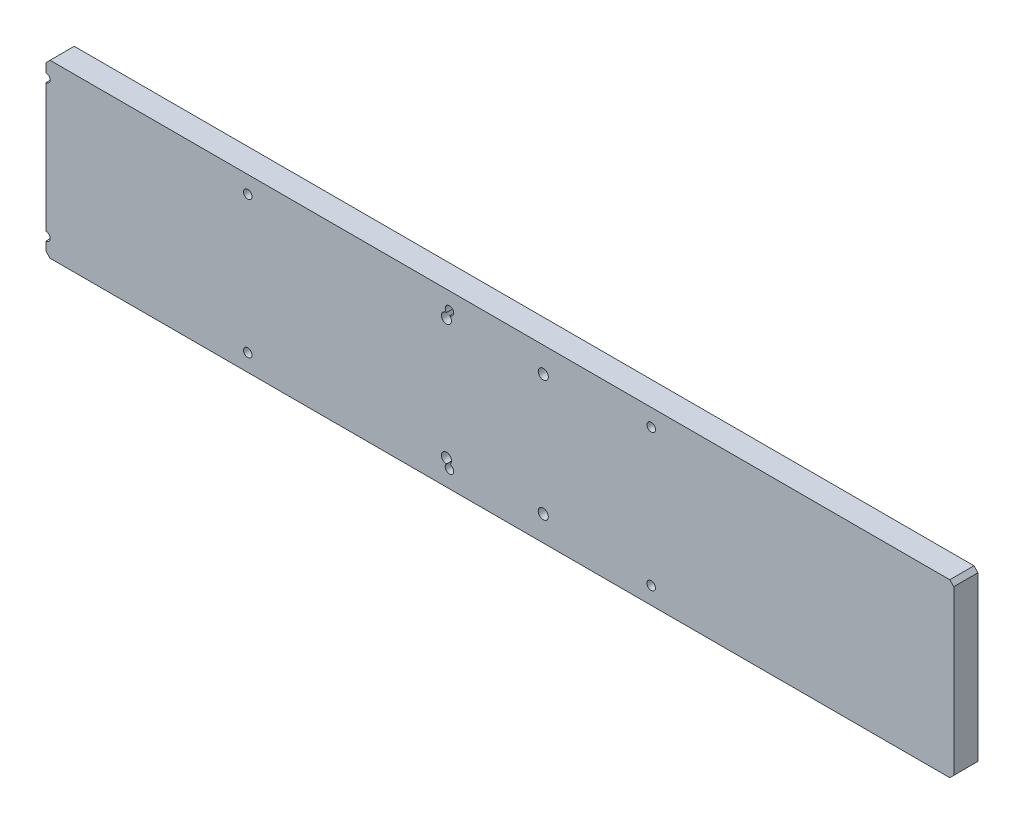
SolidWorks part; units mm, degrees
material "A6061"
ref_plane "前基準面" through (0, 0, 0) normal (0, 0, 1) x (1, 0, 0)
ref_plane "上基準面" through (0, 0, 0) normal (0, 1, 0) x (1, 0, 0)
ref_plane "右基準面" through (0, 0, 0) normal (1, 0, 0) x (0, 0, -1)
sketch "草图1" plane through (0, 0, 0) normal (0, 0, 1) x (1, 0, 0)
  line L1 (-225, -42.5) -> (225, -42.5)
  line L2 (-225, -42.5) -> (-225, 42.5)
  line L3 (-225, 42.5) -> (225, 42.5)
  line L4 (225, -42.5) -> (225, 42.5)
  line L5 (-225, -42.5) -> (225, 42.5) construction
  line L6 (-225, 42.5) -> (225, -42.5) construction
  point P0 (0, 0)
  dimension "D1" = 85
  dimension "D2" = 450
extrude "凸台-拉伸1" add sketch "草图1" along normal blind 12
sketch "草图4" plane through (0, 0, 0) normal (0, 0, -1) x (-1, 0, 0)
  line L0 (0, 0) -> (168.5016, 0) construction
  line L1 (225, 42.5) -> (225, -42.5) construction
  point P0 (26.5, 30)
  point P3 (-21.5, -30)
  point P12 (-21.5, 30)
  point P14 (26.5, -30)
  point P19 (-253.5, 30)
  point P20 (-301.5, -30)
  point P21 (-301.5, 30)
  point P22 (-253.5, -30)
  dimension "D1" = 2
  dimension "D2" = 60
  dimension "D3" = 48
  dimension "D4" = 280
  dimension "D5" = 198.5
hole_wizard "M6 螺纹孔1" positions "草图4" profile "草图5" tap size "M6" standard "GB" end condition through all
sketch "草图5" plane through (-26.5, 30, 0) normal (1, 0, 0) x (0, 1, 0)
  line L0 (0, 0) -> (0, 12)
  line L1 (0, 12) -> (2.5, 12)
  line L2 (2.5, 12) -> (2.5, 0)
  line L5 (2.5, 0) -> (0, 0)
  line L11 (0, -6.35) -> (0, 107.95) construction
  dimension "通孔螺纹孔钻头直径" = 5
  dimension "通孔螺纹孔钻头深度" = 12
cosmetic thread "孔螺纹线18" parameters "D2"=6
cosmetic thread "孔螺纹线19" parameters "D2"=6
cosmetic thread "孔螺纹线23" parameters "D2"=6
cosmetic thread "孔螺纹线24" parameters "D2"=6
hole_wizard "M5 螺纹孔1" positions "草图6" profile "草图7" tap size "M5" standard "GB" end condition through all
sketch "草图6" plane through (0, 0, 12) normal (0, 0, 1) x (1, 0, 0)
  line L0 (0, 0) -> (294.1276, 0) construction
  line L2 (225, -42.5) -> (225, 42.5) construction
  point P0 (75, 34)
  point P2 (75, -34)
  point P16 (-25, 34)
  point P17 (-25, -34)
  point P23 (-125, 34)
  point P24 (-125, -34)
  point P25 (-225, 34)
  point P26 (-225, -34)
  dimension "D1" = 68
  dimension "D2" = 150
  dimension "D4" = 100
  dimension "D3" = 4
sketch "草图7" plane through (75, 34, 12) normal (1, 0, 0) x (0, -1, 0)
  line L0 (0, 0) -> (0, 12)
  line L1 (0, 12) -> (2.1, 12)
  line L2 (2.1, 12) -> (2.1, 0)
  line L5 (2.1, 0) -> (0, 0)
  line L11 (0, -6.35) -> (0, 107.95) construction
  dimension "通孔螺纹孔钻头直径" = 4.2
  dimension "通孔螺纹孔钻头深度" = 12
cosmetic thread "孔螺蚊线1" parameters "D2"=5
cosmetic thread "孔螺蚊线2" parameters "D2"=5
cosmetic thread "孔螺蚊线5" parameters "D2"=5
cosmetic thread "孔螺蚊线6" parameters "D2"=5
cosmetic thread "孔螺蚊线7" parameters "D2"=5
cosmetic thread "孔螺蚊线8" parameters "D2"=5
cosmetic thread "孔螺蚊线11" parameters "D2"=5
cosmetic thread "孔螺蚊线12" parameters "D2"=5
hole_wizard "Ø5.0mm 暗销孔1" positions "草图8" profile "草图9" hole size "Ø5.0" standard "GB"
sketch "草图8" plane through (0, 0, 0) normal (0, 0, -1) x (-1, 0, 0)
  line L0 (-75, 34) -> (-75, -34) construction
  line L2 (225, 34) -> (225, -34) construction
  point P0 (-75, 0)
  point P14 (225, 0)
sketch "草图9" plane through (75, 0, 0) normal (1, 0, 0) x (0, 1, 0)
  line L0 (0, 0) -> (0, 6.5022)
  line L1 (0, 6.5022) -> (2.5, 5)
  line L2 (2.5, 5) -> (2.5, 0)
  line L5 (2.5, 0) -> (0, 0)
  line L10 (0, 6.5022) -> (-2.5, 5) construction
  line L11 (0, -6.35) -> (0, 107.95) construction
  dimension "孔直径" = 5
  dimension "孔深度" = 5
  dimension "导头角度" = 118
chamfer "倒角1" distance 2 angle 45 4 edges at (225, 42.5, 6) (225, -42.5, 6) (-225, 42.5, 6) (-225, -42.5, 6)
